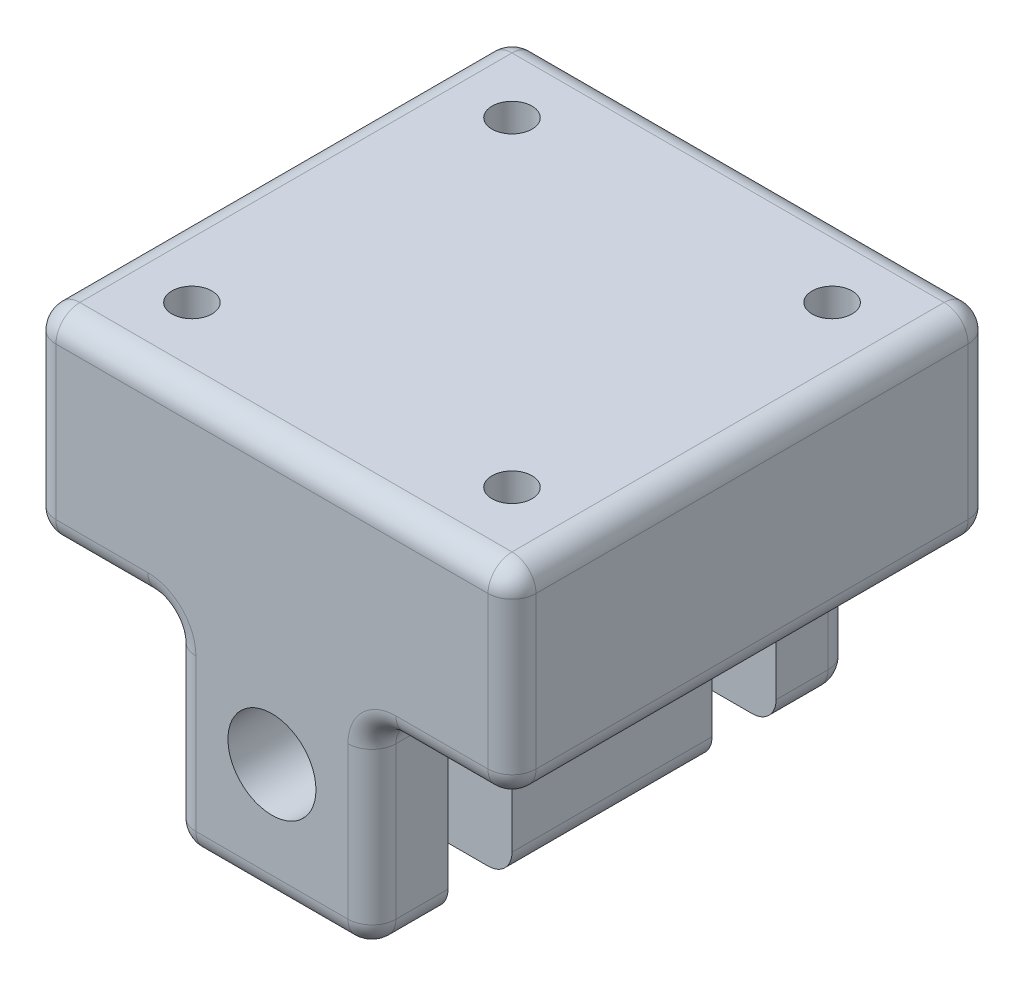
SolidWorks part; units mm, degrees
material "Beech"
ref_plane "Front Plane" through (0, 0, 0) normal (0, 0, 1) x (1, 0, 0)
ref_plane "Top Plane" through (0, 0, 0) normal (0, 1, 0) x (1, 0, 0)
ref_plane "Right Plane" through (0, 0, 0) normal (1, 0, 0) x (0, 0, -1)
sketch "Sketch1" plane through (0, 0, 0) normal (0, 0, 1) x (1, 0, 0)
  line L0 (0, 0) -> (0, 104.5883) construction
  line L1 (-12.5, 0) -> (12.5, 0)
  line L2 (-12.5, 0) -> (-12.5, 50)
  line L3 (-12.5, 50) -> (12.5, 50)
  line L4 (12.5, 0) -> (12.5, 50)
  line L5 (-30, 50) -> (30, 50)
  line L6 (-30, 50) -> (-30, 25)
  line L7 (-30, 25) -> (30, 25)
  line L8 (30, 50) -> (30, 25)
  circle A0 centre (0, 15) radius 5.5
  dimension "D5" = 15
  dimension "D6" = 11
  dimension "D1" = 60
  dimension "D2" = 25
  dimension "D3" = 25
  dimension "D4" = 50
extrude "Boss-Extrude1" add sketch "Sketch1" along normal mid plane 60 contours L1 L0 A0 L7 L2 | L0 L1 L4 L7 A0 | L8 L5 L4 L7 | L0 L7 L4 L5 | L7 L0 L3 L2 | L6 L7 L2 L5
fillet "Fillet1" radius 3 24 edges at (21.25, 25, -30) (-21.25, 25, -30) (12.5, 12.5, -30) (12.5, 12.5, 30) (-12.5, 12.5, -30) (-12.5, 12.5, 30) (30, 50, 0) (0, 50, -30) (0, 50, 30) (-30, 50, 0) (0, 0, -30) (-12.5, 0, 0) (0, 0, 30) (12.5, 0, 0) (21.25, 25, 30) (-21.25, 25, 30) (-30, 25, 0) (30, 25, 0) (-12.5, 25, 0) (12.5, 25, 0) (30, 37.5, -30) (30, 37.5, 30) (-30, 37.5, -30) (-30, 37.5, 30)
sketch "Sketch2" plane through (0, 0, 0) normal (0, -1, 0) x (1, 0, 0)
  line L0 (-34.7143, 0) -> (37.6849, 0) construction
  line L1 (0, 0) -> (0, 24.1472) construction
  line L2 (12.5, 20.5) -> (-12.5, 20.5)
  line L3 (12.5, 20.5) -> (12.5, 12.5)
  line L4 (12.5, 12.5) -> (-12.5, 12.5)
  line L5 (-12.5, 20.5) -> (-12.5, 12.5)
  line L6 (12.5, -12.5) -> (-12.5, -12.5)
  line L7 (12.5, -12.5) -> (12.5, -20.5)
  line L8 (12.5, -20.5) -> (-12.5, -20.5)
  line L9 (-12.5, -12.5) -> (-12.5, -20.5)
  dimension "D1" = 8
  dimension "D2" = 25
  dimension "D3" = 25
extrude "Cut-Extrude1" cut sketch "Sketch2" against normal blind 23
sketch "Sketch3" plane through (0, 25, 0) normal (0, -1, 0) x (1, 0, 0)
  circle A0 centre (20, 20) radius 2.5
  circle A1 centre (20, -20) radius 2.5
  circle A2 centre (-20, -20) radius 2.5
  circle A3 centre (-20, 20) radius 2.5
  point P12 (0, 0)
  dimension "D1" = 5
  dimension "D2" = 20
  dimension "D3" = 20
  dimension "D4" = 4
extrude "Cut-Extrude2" cut sketch "Sketch3" against normal through all
